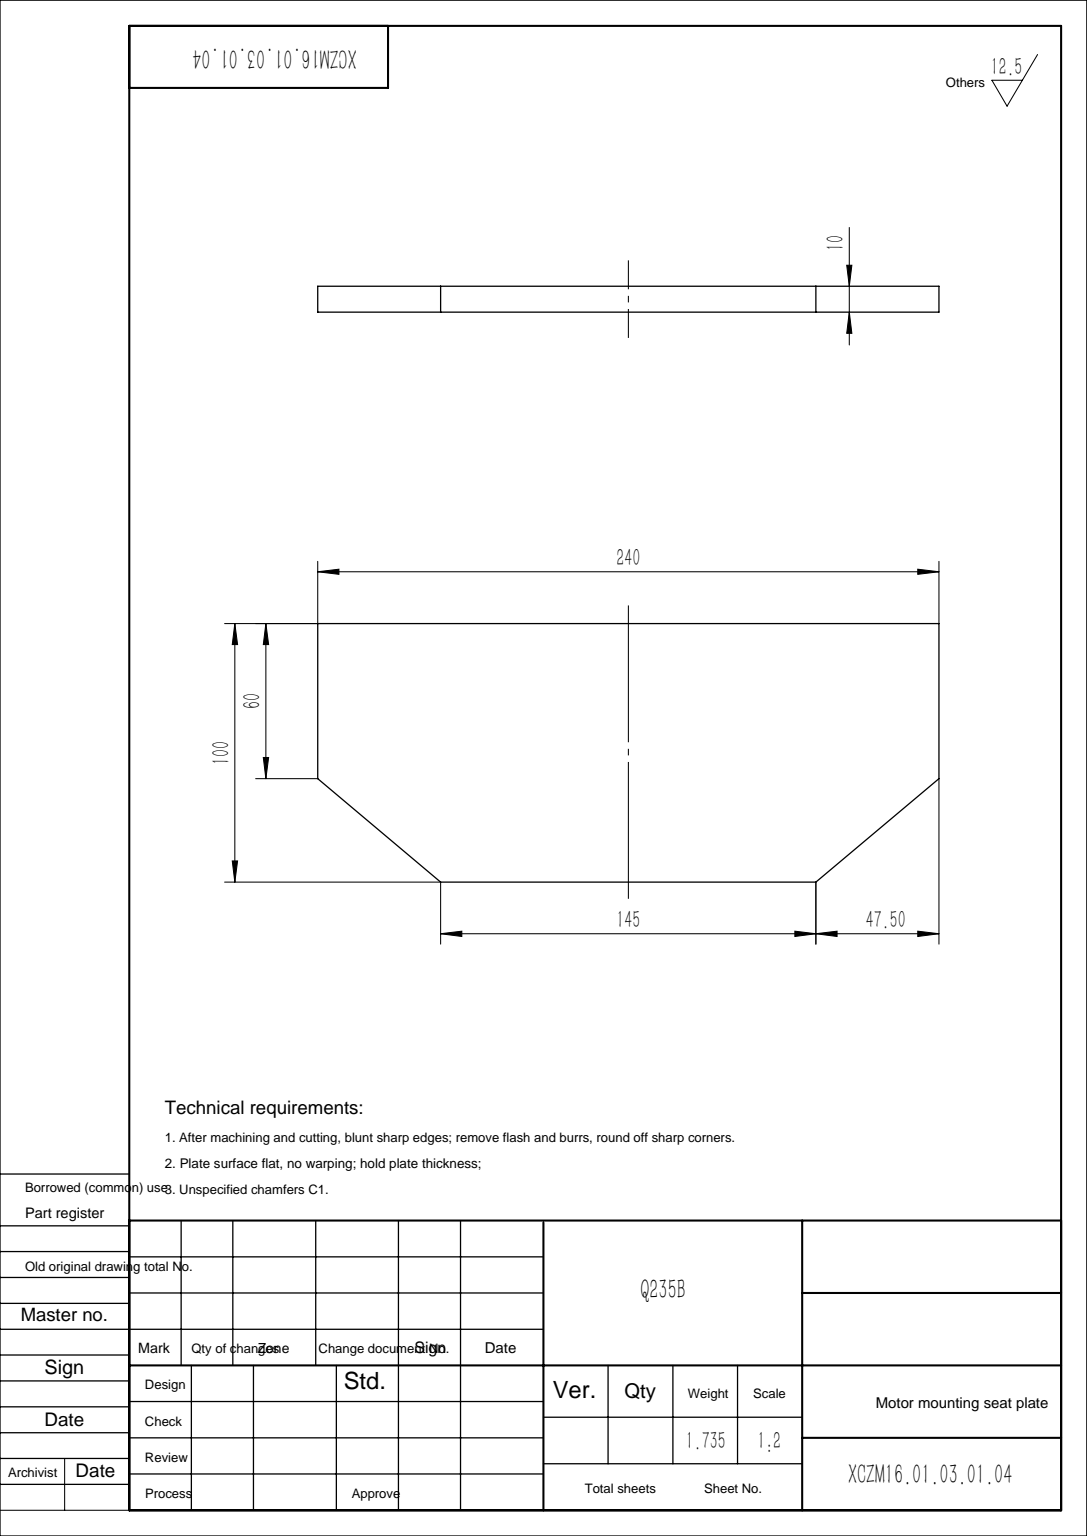
SolidWorks part; units mm, degrees
material "XRAAT"
ref_plane "前视基准面" through (0, 0, 0) normal (0, 0, 1) x (1, 0, 0)
ref_plane "上视基准面" through (0, 0, 0) normal (0, 1, 0) x (1, 0, 0)
ref_plane "右视基准面" through (0, 0, 0) normal (1, 0, 0) x (0, 0, -1)
sketch "草图1" plane through (0, 0, 0) normal (0, 0, 1) x (1, 0, 0)
  line L0 (120, 0) -> (-120, 0)
  line L1 (-120, 0) -> (-120, -60)
  line L2 (-120, -60) -> (-72.5, -100)
  line L3 (-72.5, -100) -> (72.5, -100)
  line L4 (0, -100) -> (0, 0) construction
  line L5 (120, -60) -> (72.5, -100)
  line L6 (120, 0) -> (120, -60)
  dimension "D1" = 240
  dimension "D2" = 145
  dimension "D3" = 100
  dimension "D4" = 60
extrude "凸台-拉伸1" add sketch "草图1" along normal blind 10
